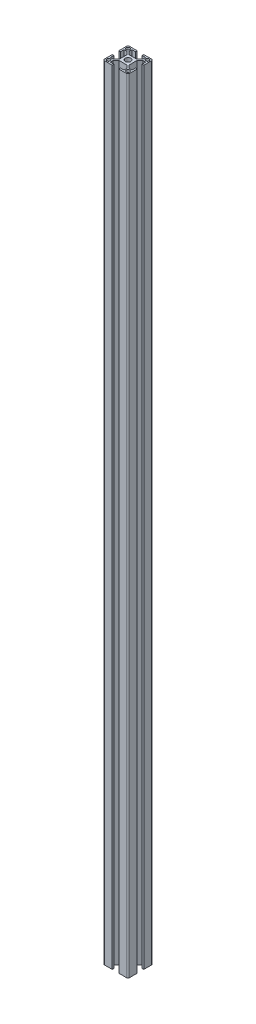
SolidWorks part; units mm, degrees
ref_plane "前视基准面" through (0, 0, 0) normal (0, 0, 1) x (1, 0, 0)
ref_plane "上视基准面" through (0, 0, 0) normal (0, 1, 0) x (1, 0, 0)
ref_plane "右视基准面" through (0, 0, 0) normal (1, 0, 0) x (0, 0, -1)
sketch "草图1" plane through (0, 0, 0) normal (0, 1, 0) x (1, 0, 0)
  line L44 (6.75, -28) -> (11, -28)
  line L45 (11, -28) -> (11, -30)
  line L46 (11, -30) -> (2, -30)
  line L47 (0, -28) -> (0, -19)
  line L48 (0, -19) -> (2, -19)
  line L49 (2, -19) -> (2, -23.25)
  line L50 (28, -30) -> (19, -30)
  line L51 (19, -30) -> (19, -28)
  line L52 (23.25, -28) -> (23.25, -24.6642)
  line L53 (19, -28) -> (23.25, -28)
  line L54 (30, -19) -> (30, -28)
  line L55 (28, -19) -> (30, -19)
  line L56 (28, -23.25) -> (28, -19)
  line L57 (24.6642, -23.25) -> (28, -23.25)
  line L58 (21, -19.5858) -> (24.6642, -23.25)
  line L59 (23.25, -24.6642) -> (19.5858, -21)
  line L60 (6.75, -24.6642) -> (6.75, -28)
  line L61 (2, -23.25) -> (5.3358, -23.25)
  line L62 (5.3358, -23.25) -> (9, -19.5858)
  line L63 (10.4142, -21) -> (6.75, -24.6642)
  line L64 (19.5858, -21) -> (10.4142, -21)
  line L65 (9, -19.5858) -> (9, -10.4142)
  line L66 (21, -10.4142) -> (21, -19.5858)
  line L67 (30, -11) -> (28, -11)
  line L68 (28, -11) -> (28, -6.75)
  line L69 (28, -6.75) -> (24.6642, -6.75)
  line L70 (24.6642, -6.75) -> (21, -10.4142)
  line L71 (19.5858, -9) -> (23.25, -5.3358)
  line L72 (10.4142, -9) -> (19.5858, -9)
  line L73 (6.75, -5.3358) -> (10.4142, -9)
  line L74 (9, -10.4142) -> (5.3358, -6.75)
  line L75 (2, -11) -> (0, -11)
  line L76 (2, -6.75) -> (2, -11)
  line L77 (5.3358, -6.75) -> (2, -6.75)
  line L78 (6.75, -2) -> (6.75, -5.3358)
  line L79 (23.25, -5.3358) -> (23.25, -2)
  line L80 (23.25, -2) -> (19, -2)
  line L81 (19, -2) -> (19, 0)
  line L82 (11, 0) -> (11, -2)
  line L83 (11, -2) -> (6.75, -2)
  line L84 (30, -2) -> (30, -11)
  line L85 (19, 0) -> (28, 0)
  line L86 (2, 0) -> (11, 0)
  line L87 (0, -11) -> (0, -2)
  line L88 (0, -15) -> (30, -15) construction
  line L89 (15, -30) -> (15, 0) construction
  line L90 (0, 0) -> (30, -30) construction
  line L91 (0, -30) -> (30, 0) construction
  arc A9 (0, -28) -> (2, -30) centre (2, -28) ccw
  circle A10 centre (3.375, -26.625) radius 2.1
  circle A11 centre (26.625, -26.625) radius 2.1
  arc A12 (28, -30) -> (30, -28) centre (28, -28) ccw
  circle A13 centre (15, -15) radius 3.4
  circle A14 centre (3.375, -3.375) radius 2.1
  circle A15 centre (26.625, -3.375) radius 2.1
  arc A16 (30, -2) -> (28, 0) centre (28, -2) ccw
  arc A17 (2, 0) -> (0, -2) centre (2, -2) ccw
  dimension "D2" = 15
  dimension "D5" = 6.8
  dimension "D8" = 6
  dimension "D11" = 23.25
  dimension "D12" = 3.375
  dimension "D13" = 23.25
  dimension "D14" = 4.2
  dimension "D15" = 2
  dimension "D16" = 2
  dimension "D23" = 2
  dimension "D24" = 2
  dimension "D1" = 15
  dimension "D3" = 45
  dimension "D4" = 45
  dimension "D6" = 30
  dimension "D7" = 30
  dimension "D9" = 12
  dimension "D10" = 3.375
  dimension "D17" = 11
  dimension "D18" = 8
  dimension "D19" = 2
  dimension "D20" = 2
  dimension "D21" = 11
  dimension "D22" = 8
  dimension "D25" = 2
  dimension "D26" = 2
  dimension "D27" = 6.75
  dimension "D28" = 16.5
  dimension "D29" = 6.75
  dimension "D30" = 16.5
  dimension "D31" = 12
  dimension "D32" = 6
  dimension "D33" = 2
  dimension "D34" = 1
  dimension "D35" = 2
  dimension "D36" = 1
extrude "拉伸1" add sketch "草图1" along normal blind 940
